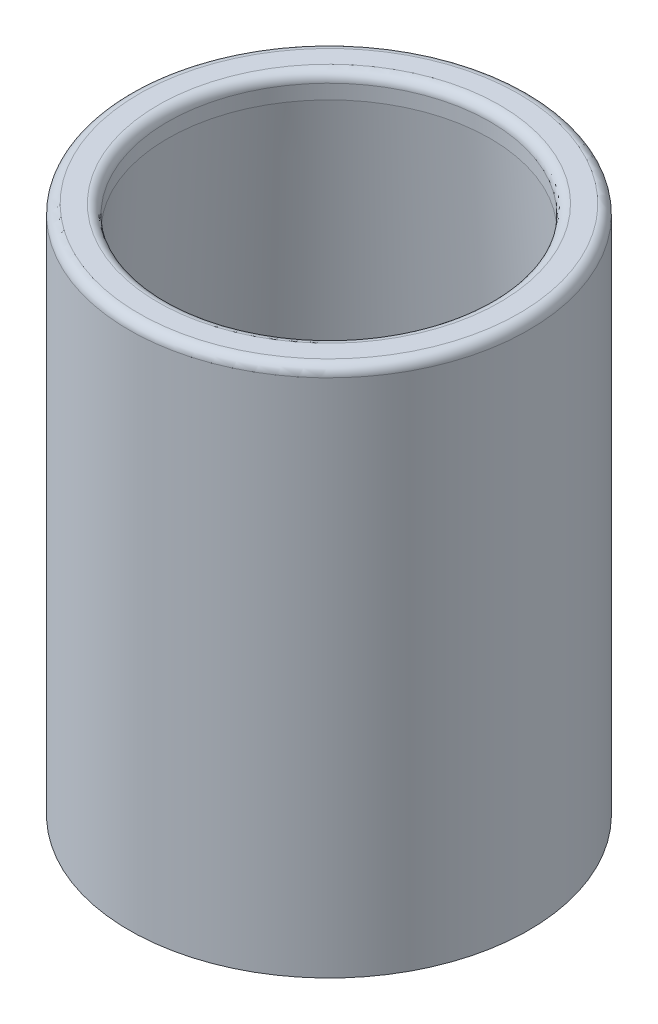
SolidWorks part; units mm, degrees
material "SPHC"
ref_plane "Front Plane" through (0, 0, 0) normal (0, 0, 1) x (1, 0, 0)
ref_plane "Top Plane" through (0, 0, 0) normal (0, 1, 0) x (1, 0, 0)
ref_plane "Right Plane" through (0, 0, 0) normal (1, 0, 0) x (0, 0, -1)
sketch "Sketch1" plane through (0, 0, 0) normal (0, 0, 1) x (1, 0, 0)
  line L0 (0, 0) -> (0, 110) construction
  line L1 (41.5, 0) -> (41.5, 108)
  line L2 (39.5, 110) -> (35.5, 110)
  line L3 (33.5, 108) -> (33.5, 105)
  line L4 (41.5, 0) -> (33.5, 105)
  arc A0 (35.5, 110) -> (33.5, 108) centre (35.5, 108) ccw
  arc A1 (41.5, 108) -> (39.5, 110) centre (39.5, 108) ccw
  point P8 (33.5, 110)
  point P13 (41.5, 110)
  dimension "D5" = 2
  dimension "D1" = 41.5
  dimension "D2" = 110
  dimension "D3" = 8
  dimension "D4" = 5
revolve "Revolve-Thin1" add sketch "Sketch1" angle 360 about L0 wall 1
